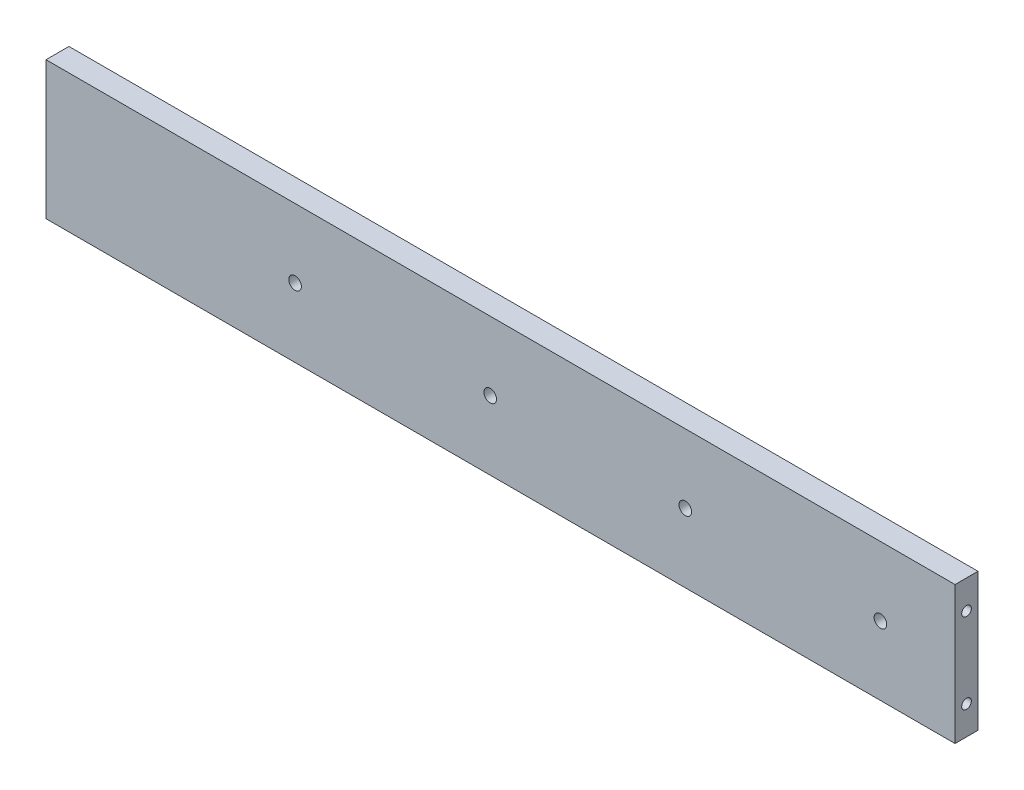
SolidWorks part; units mm, degrees
ref_plane "Front Plane" through (0, 0, 0) normal (0, 0, 1) x (1, 0, 0)
ref_plane "Top Plane" through (0, 0, 0) normal (0, 1, 0) x (1, 0, 0)
ref_plane "Right Plane" through (0, 0, 0) normal (1, 0, 0) x (0, 0, -1)
sketch "Sketch1" plane through (0, 0, 0) normal (0, 0, 1) x (1, 0, 0)
  line L1 (-198, 30) -> (198, 30)
  line L2 (-198, 30) -> (-198, -30)
  line L3 (-198, -30) -> (198, -30)
  line L4 (198, 30) -> (198, -30)
  line L5 (-198, 30) -> (198, -30) construction
  line L6 (-198, -30) -> (198, 30) construction
  point P0 (0, 0)
  dimension "D1" = 396
  dimension "D2" = 60
extrude "Boss-Extrude1" add sketch "Sketch1" along normal blind 10
hole_wizard "Hole size per socket head cap screw type 1" positions "Sketch3" profile "Sketch2" counterbore size "M5" standard "Gb" end condition through all
sketch "Sketch3" plane through (0, 0, 0) normal (0, 0, -1) x (-1, 0, 0)
  point P0 (89.5, 0)
  point P3 (4.5, 0)
  point P6 (-80.5, 0)
  point P9 (-165.5, 0)
sketch "Sketch2" plane through (-89.5, 0, 0) normal (1, 0, 0) x (0, 1, 0)
  line L0 (0, 0) -> (0, 10)
  line L1 (0, 10) -> (2.75, 10)
  line L3 (2.75, 10) -> (2.75, 5.7)
  line L4 (2.75, 5.7) -> (5, 5.7)
  line L5 (5, 5.7) -> (5, 0)
  line L7 (5, 0) -> (0, 0)
  line L11 (0, -6.35) -> (0, 107.95) construction
  dimension "通孔孔直径" = 5.5
  dimension "通孔孔深度" = 10
  dimension "柱形沉头孔直径" = 10
  dimension "柱形沉头孔深度" = 5.7
hole_wizard "M5 Tapped Hole1" positions "Sketch5" profile "Sketch4" tap size "M5" standard "Gb"
sketch "Sketch5" plane through (-198, 0, 0) normal (-1, 0, 0) x (0, 0, 1)
  line L0 (0, 0) -> (23.4439, 0) construction
  line L2 (5, 30) -> (5, 36.7094) construction
  line L3 (10, 30) -> (0, 30) construction
  point P0 (5, 17.5)
  point P2 (5, -17.5)
  dimension "D1" = 35
sketch "Sketch4" plane through (-198, 17.5, 5) normal (0, 1, 0) x (0, 0, 1)
  line L0 (0, 0) -> (0, 13.6618)
  line L1 (0, 13.6618) -> (2.1, 12.4)
  line L2 (2.1, 12.4) -> (2.1, 0)
  line L5 (2.1, 0) -> (0, 0)
  line L10 (0, 13.6618) -> (-2.1, 12.4) construction
  line L11 (0, -6.35) -> (0, 107.95) construction
  dimension "螺纹孔钻头直径" = 4.2
  dimension "螺纹孔钻头深度" = 12.4
  dimension "导头角度" = 118
cosmetic thread "Cosmetic Thread 1" parameters "D1"=10, "D2"=5
cosmetic thread "Cosmetic Thread 2" parameters "D1"=10, "D2"=5
mirror "Mirror1" about plane through (0, 0, 0) normal (1, 0, 0) of "M5 Tapped Hole1"
